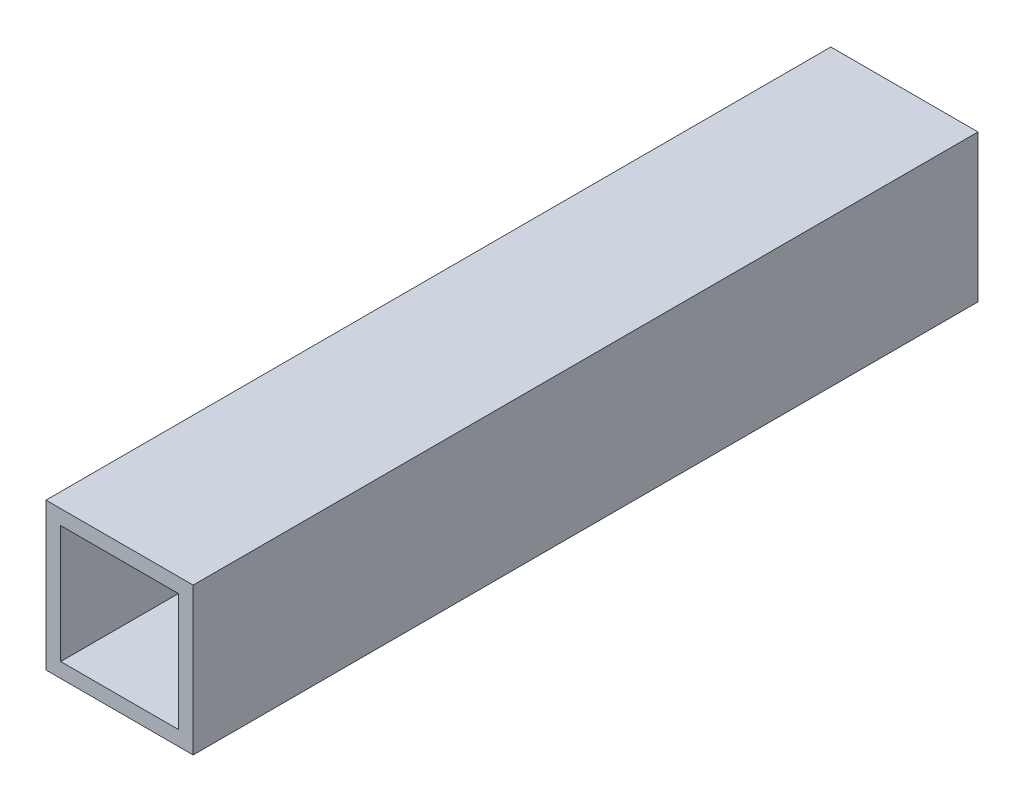
SolidWorks part; units mm, degrees
ref_plane "前视基准面" through (0, 0, 0) normal (0, 0, 1) x (1, 0, 0)
ref_plane "上视基准面" through (0, 0, 0) normal (0, 1, 0) x (1, 0, 0)
ref_plane "右视基准面" through (0, 0, 0) normal (1, 0, 0) x (0, 0, -1)
other "Configuration Table"
sketch "草图1" plane through (0, 0, 0) normal (0, 0, 1) x (1, 0, 0)
  line L0 (-15, -15) -> (15, -15)
  line L1 (15, -15) -> (15, 15)
  line L2 (15, 15) -> (-15, 15)
  line L3 (-15, 15) -> (-15, -15)
  line L4 (-12, -12) -> (12, -12)
  line L5 (12, -12) -> (12, 12)
  line L6 (12, 12) -> (-12, 12)
  line L7 (-12, 12) -> (-12, -12)
  point P0 (0, 0)
  dimension "D1" = 3
  dimension "D2" = 15
  dimension "D3" = 27
  dimension "D4" = 30
  dimension "D5" = 3
  dimension "D6" = 15
  dimension "D7" = 27
  dimension "D8" = 30
extrude "凸台-拉伸1" add sketch "草图1" against normal mid plane 160
